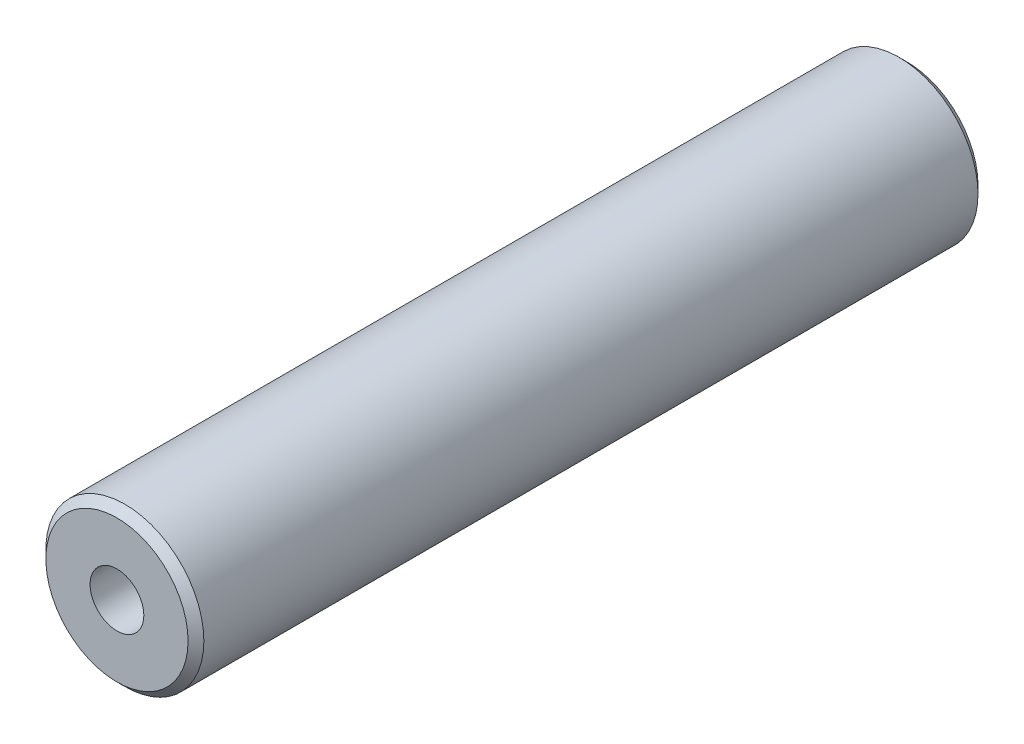
SolidWorks part; units mm, degrees
material "-"
ref_plane "Front Plane" through (0, 0, 0) normal (0, 0, 1) x (1, 0, 0)
ref_plane "Top Plane" through (0, 0, 0) normal (0, 1, 0) x (1, 0, 0)
ref_plane "Right Plane" through (0, 0, 0) normal (1, 0, 0) x (0, 0, -1)
sketch "Sketch1" plane through (0, 0, 0) normal (0, 0, 1) x (1, 0, 0)
  circle A0 centre (0, 0) radius 10
  dimension "D1" = 20
extrude "Boss-Extrude1" add sketch "Sketch1" along normal blind 100
hole_wizard "M8 Tapped Hole1" positions "Sketch3" profile "Sketch2" tap size "M8" standard "GB"
sketch "Sketch3" plane through (0, 0, 100) normal (0, 0, 1) x (1, 0, 0)
  point P0 (0, 0)
sketch "Sketch2" plane through (0, 0, 100) normal (1, 0, 0) x (0, -1, 0)
  line L0 (0, 0) -> (0, 24.2929)
  line L1 (0, 24.2929) -> (3.4, 22.25)
  line L2 (3.4, 22.25) -> (3.4, 0)
  line L5 (3.4, 0) -> (0, 0)
  line L10 (0, 24.2929) -> (-3.4, 22.25) construction
  line L11 (0, -6.35) -> (0, 107.95) construction
  dimension "螺纹孔钻头直径" = 6.8
  dimension "螺纹孔钻头深度" = 22.25
  dimension "导头角度" = 118
cosmetic thread "Cosmetic thread 1" parameters "D1"=16, "D2"=8
chamfer "Chamfer1" distance 1 angle 45 1 edges at (10, 0, 100)
chamfer "Chamfer3" distance 1 angle 45 1 edges at (10, 0, 0)
hole_wizard "M8 Tapped Hole2" positions "Sketch5" profile "Sketch4" tap size "M8" standard "GB"
sketch "Sketch5" plane through (0, 0, 0) normal (0, 0, -1) x (-1, 0, 0)
  point P0 (0, 0)
  dimension "D1" = 0
sketch "Sketch4" plane through (0, 0, 0) normal (1, 0, 0) x (0, 1, 0)
  line L0 (0, 0) -> (0, 24.2929)
  line L1 (0, 24.2929) -> (3.4, 22.25)
  line L2 (3.4, 22.25) -> (3.4, 0)
  line L5 (3.4, 0) -> (0, 0)
  line L10 (0, 24.2929) -> (-3.4, 22.25) construction
  line L11 (0, -6.35) -> (0, 107.95) construction
  dimension "螺纹孔钻头直径" = 6.8
  dimension "螺纹孔钻头深度" = 22.25
  dimension "导头角度" = 118
cosmetic thread "Cosmetic thread 2" parameters "D1"=16, "D2"=8
